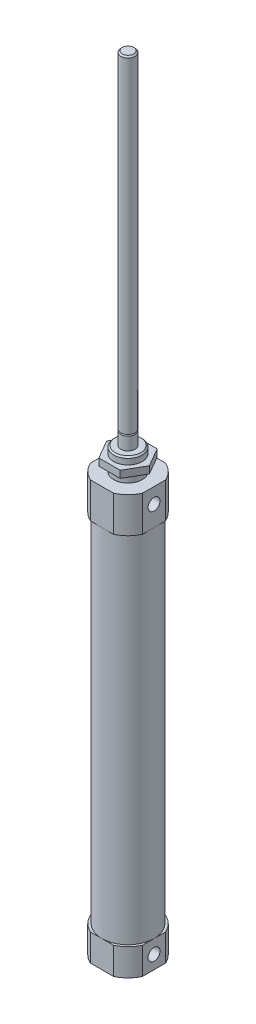
from build123d import *

# Parameters (mm, degrees)
BOSS_EXTRUDE1_DEPTH   = 12.5
SKETCH3_R             = 9.15
BOSS_EXTRUDE2_DEPTH   = 125
BOSS_EXTRUDE3_START   = 9.5
BOSS_EXTRUDE3_DEPTH   = 9.5
SKETCH5_R             = 5
BOSS_EXTRUDE4_DEPTH   = 8
SKETCH6_R             = 2.5
BOSS_EXTRUDE5_DEPTH   = 5
CHAMFER1_SIZE         = 0.5
SKETCH8_R             = 2.5
BOSS_EXTRUDE6_DEPTH   = 115
CHAMFER2_SIZE         = 0.5
BOSS_EXTRUDE7_DEPTH   = 2.5
CHAMFER4_SIZE         = 0.5
M5_TAPPED_HOLE1_D     = 4.2
M5_TAPPED_HOLE1_DEPTH = 14
M5_TAPPED_HOLE1_TIP   = 1.2618073


with BuildPart() as part:
    # Sketch1 → Boss-Extrude1 (new body)
    with BuildSketch(Plane(origin=(0, 0, 0), x_dir=(1, 0, 0), z_dir=(0, 1, 0))):
        with BuildLine():
            Line((-4.034538387, 9.15), (4.034538387, 9.15))
            ThreePointArc((4.034538387, 9.15), (7.071067812, 7.071067812), (9.15, 4.034538387))
            Line((9.15, 4.034538387), (9.15, -4.034538387))
            ThreePointArc((9.15, -4.034538387), (7.071067812, -7.071067812), (4.034538387, -9.15))
            Line((4.034538387, -9.15), (-4.034538387, -9.15))
            ThreePointArc((-4.034538387, -9.15), (-7.071067812, -7.071067812), (-9.15, -4.034538387))
            Line((-9.15, -4.034538387), (-9.15, 4.034538387))
            ThreePointArc((-9.15, 4.034538387), (-7.071067812, 7.071067812), (-4.034538387, 9.15))
        make_face()
    extrude(amount=BOSS_EXTRUDE1_DEPTH)

    # Sketch3 → Boss-Extrude2 (add)
    with BuildSketch(Plane.XZ):
        with Locations(Location((0, 0, 0), (0, 0, 270))):
            Circle(SKETCH3_R)
    extrude(amount=BOSS_EXTRUDE2_DEPTH)

    # Sketch4 → Boss-Extrude3 (add)
    with BuildSketch(Plane.XZ.offset(125).offset(BOSS_EXTRUDE3_START)):
        with BuildLine():
            Line((-4.034538387, 9.15), (4.034538387, 9.15))
            ThreePointArc((4.034538387, 9.15), (7.071067812, 7.071067812), (9.15, 4.034538387))
            Line((9.15, 4.034538387), (9.15, -4.034538387))
            ThreePointArc((9.15, -4.034538387), (7.071067812, -7.071067812), (4.034538387, -9.15))
            Line((4.034538387, -9.15), (-4.034538387, -9.15))
            ThreePointArc((-4.034538387, -9.15), (-7.071067812, -7.071067812), (-9.15, -4.034538387))
            Line((-9.15, -4.034538387), (-9.15, 4.034538387))
            ThreePointArc((-9.15, 4.034538387), (-7.071067812, 7.071067812), (-4.034538387, 9.15))
        make_face()
    extrude(amount=-BOSS_EXTRUDE3_DEPTH)

    # Sketch5 → Boss-Extrude4 (add)
    with BuildSketch(Plane(origin=(0, 12.5, 0), x_dir=(1, 0, 0), z_dir=(0, 1, 0))):
        with Locations(Location((0, 0, 0), (0, 0, 270))):
            Circle(SKETCH5_R)
    extrude(amount=BOSS_EXTRUDE4_DEPTH)

    # Sketch6 → Boss-Extrude5 (add)
    with BuildSketch(Plane(origin=(0, 20.5, 0), x_dir=(1, 0, 0), z_dir=(0, 1, 0))):
        with Locations(Location((0, 0, 0), (0, 0, 270))):
            Circle(SKETCH6_R)
    extrude(amount=BOSS_EXTRUDE5_DEPTH)

    # Chamfer1
    chamfer1_edges = [part.edges().sort_by_distance(p)[0] for p in [
        (0, 25.5, -2.5),
    ]]
    chamfer(chamfer1_edges, length=CHAMFER1_SIZE)

    # Sketch8 → Boss-Extrude6 (add)
    with BuildSketch(Plane(origin=(0, 25.5, 0), x_dir=(1, 0, 0), z_dir=(0, 1, 0))):
        with Locations(Location((0, 0, 0), (0, 0, 270))):
            Circle(SKETCH8_R)
    extrude(amount=BOSS_EXTRUDE6_DEPTH)

    # Chamfer2
    chamfer2_edges = [part.edges().sort_by_distance(p)[0] for p in [
        (0, 20.5, -5),
    ]]
    chamfer(chamfer2_edges, length=CHAMFER2_SIZE)

    # Sketch9 → Boss-Extrude7 (add)
    with BuildSketch(Plane(origin=(0, 15.5, 0), x_dir=(1, 0, 0), z_dir=(0, 1, 0))):
        Polygon((7.505553499, 0), (3.75277675, 6.5), (-3.75277675, 6.5), (-7.505553499, 0), (-3.75277675, -6.5), (3.75277675, -6.5), align=None)
    extrude(amount=BOSS_EXTRUDE7_DEPTH)

    # Chamfer4
    chamfer4_edges = [part.edges().sort_by_distance(p)[0] for p in [
        (0, 140.5, -2.5),
    ]]
    chamfer(chamfer4_edges, length=CHAMFER4_SIZE)

    # M5 Tapped Hole1
    with Locations(Plane(origin=(9.15, 0, 0), x_dir=(0, 0, -1), z_dir=(1, 0, 0))):
        with Locations((0, 7.109181896), (0, -129.804166053)):
            Hole(M5_TAPPED_HOLE1_D / 2, depth=M5_TAPPED_HOLE1_DEPTH)
            with Locations((0, 0, -(M5_TAPPED_HOLE1_DEPTH + M5_TAPPED_HOLE1_TIP / 2))):  # 118° drill point
                Cone(0, M5_TAPPED_HOLE1_D / 2, M5_TAPPED_HOLE1_TIP, mode=Mode.SUBTRACT)


solid = part.part
